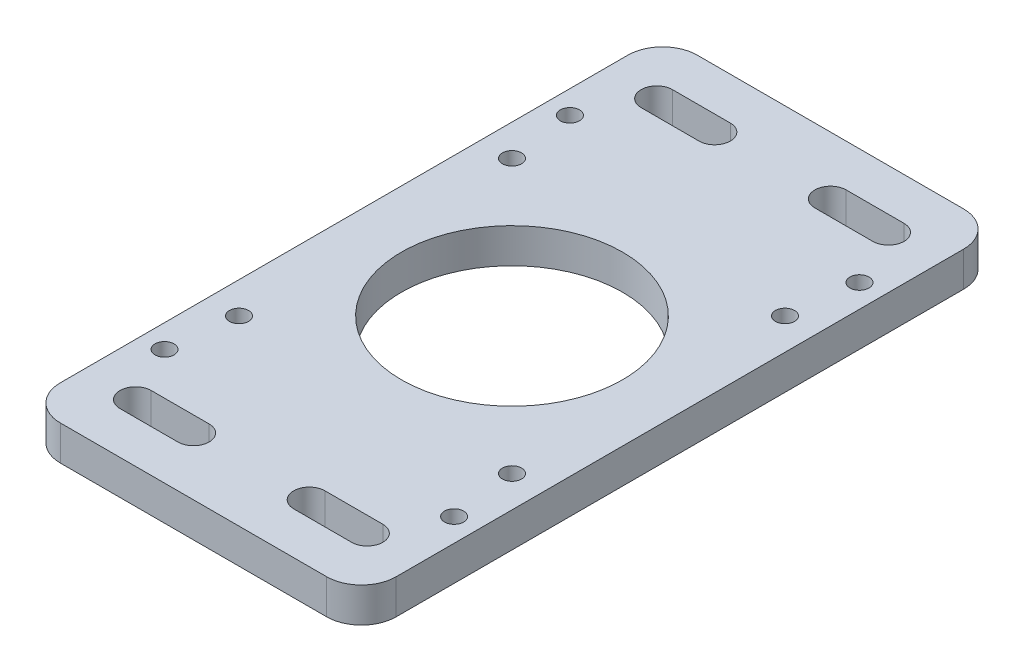
from build123d import *

# Parameters (mm, degrees)
SKETCH1_R             = 19.1
BOSS_EXTRUDE1_DEPTH   = 6
M4_TAPPED_HOLE1_D     = 3.3
M4_TAPPED_HOLE1_DEPTH = 10.1
M4_TAPPED_HOLE1_TIP   = 0.991420021
CUT_EXTRUDE1_DEPTH    = 63.465990747
M4_TAPPED_HOLE2_D     = 3.3
M4_TAPPED_HOLE2_DEPTH = 10.1
M4_TAPPED_HOLE2_TIP   = 0.991420021


with BuildPart() as part:
    # Sketch1 → Boss-Extrude1 (new body)
    with BuildSketch(Plane(origin=(0, 0, 0), x_dir=(1, 0, 0), z_dir=(0, 1, 0))):
        with BuildLine():
            Line((-23, 55), (23, 55))
            ThreePointArc((23, 55), (27.242640687, 53.242640687), (29, 49))
            Line((29, 49), (29, -49))
            ThreePointArc((29, -49), (27.242640687, -53.242640687), (23, -55))
            Line((23, -55), (-23, -55))
            ThreePointArc((-23, -55), (-27.242640687, -53.242640687), (-29, -49))
            Line((-29, -49), (-29, 49))
            ThreePointArc((-29, 49), (-27.242640687, 53.242640687), (-23, 55))
        make_face()
        with Locations(Location((0, 0, 0), (0, 0, 270))):
            Circle(SKETCH1_R, mode=Mode.SUBTRACT)
    extrude(amount=BOSS_EXTRUDE1_DEPTH)

    # M4 Tapped Hole1
    with Locations(Plane(origin=(0, 6, 0), x_dir=(1, 0, 0), z_dir=(0, 1, 0))):
        with Locations((-23.57, 23.57), (23.57, 23.57), (23.57, -23.57), (-23.57, -23.57)):
            Hole(M4_TAPPED_HOLE1_D / 2, depth=M4_TAPPED_HOLE1_DEPTH)
            with Locations((0, 0, -(M4_TAPPED_HOLE1_DEPTH + M4_TAPPED_HOLE1_TIP / 2))):  # 118° drill point
                Cone(0, M4_TAPPED_HOLE1_D / 2, M4_TAPPED_HOLE1_TIP, mode=Mode.SUBTRACT)

    # Sketch4 → Cut-Extrude1 (cut, through all)
    with BuildSketch(Plane.XZ):
        with BuildLine():
            Line((-20, 47.7), (-10, 47.7))
            ThreePointArc((-10, 47.7), (-7.3, 45), (-10, 42.3))
            Line((-10, 42.3), (-20, 42.3))
            ThreePointArc((-20, 42.3), (-22.7, 45), (-20, 47.7))
        make_face()
        with BuildLine():
            Line((20, 47.7), (10, 47.7))
            ThreePointArc((10, 47.7), (7.3, 45), (10, 42.3))
            Line((10, 42.3), (20, 42.3))
            ThreePointArc((20, 42.3), (22.7, 45), (20, 47.7))
        make_face()
        with BuildLine():
            Line((-20, -47.7), (-10, -47.7))
            ThreePointArc((-10, -47.7), (-7.3, -45), (-10, -42.3))
            Line((-10, -42.3), (-20, -42.3))
            ThreePointArc((-20, -42.3), (-22.7, -45), (-20, -47.7))
        make_face()
        with BuildLine():
            Line((20, -47.7), (10, -47.7))
            ThreePointArc((10, -47.7), (7.3, -45), (10, -42.3))
            Line((10, -42.3), (20, -42.3))
            ThreePointArc((20, -42.3), (22.7, -45), (20, -47.7))
        make_face()
    extrude(amount=-CUT_EXTRUDE1_DEPTH, mode=Mode.SUBTRACT)

    # M4 Tapped Hole2
    with Locations(Plane(origin=(0, 0, 0), x_dir=(-1, 0, 0), z_dir=(0, -1, 0))):
        with Locations((25, -35), (25, 35), (-25, 35), (-25, -35)):
            Hole(M4_TAPPED_HOLE2_D / 2, depth=M4_TAPPED_HOLE2_DEPTH)
            with Locations((0, 0, -(M4_TAPPED_HOLE2_DEPTH + M4_TAPPED_HOLE2_TIP / 2))):  # 118° drill point
                Cone(0, M4_TAPPED_HOLE2_D / 2, M4_TAPPED_HOLE2_TIP, mode=Mode.SUBTRACT)


solid = part.part
